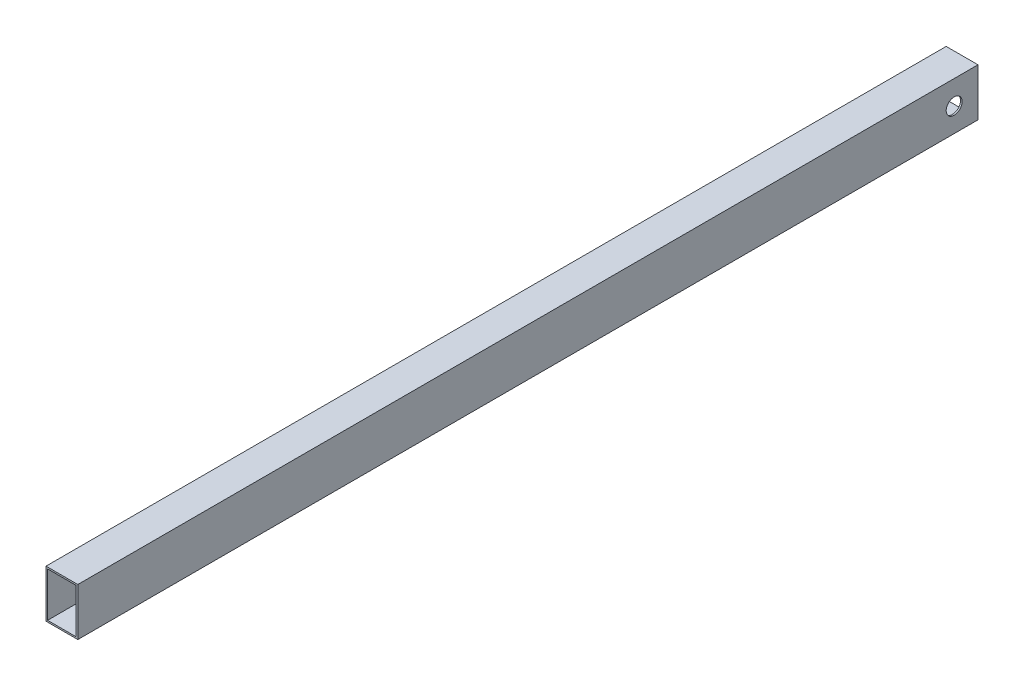
from build123d import *

# Parameters (mm, degrees)
SKETCH1_W           = 20
SKETCH1_H           = 30
SKETCH1_W_2         = 18
SKETCH1_H_2         = 28
BOSS_EXTRUDE1_DEPTH = 566
SKETCH4_R           = 5
CUT_EXTRUDE1_DEPTH  = 568.147247194


with BuildPart() as part:
    # Sketch1 → Boss-Extrude1 (new body)
    with BuildSketch(Plane.XY):
        with Locations((10, -15)):
            Rectangle(SKETCH1_W, SKETCH1_H)
        with Locations((10, -15)):
            Rectangle(SKETCH1_W_2, SKETCH1_H_2, mode=Mode.SUBTRACT)
    extrude(amount=BOSS_EXTRUDE1_DEPTH)

    # Sketch4 → Cut-Extrude1 (cut, through all)
    with BuildSketch(Plane.ZY):
        with Locations(Location((15, -15, 0), (0, 0, 270))):
            Circle(SKETCH4_R)
    extrude(amount=-CUT_EXTRUDE1_DEPTH, mode=Mode.SUBTRACT)


solid = part.part
